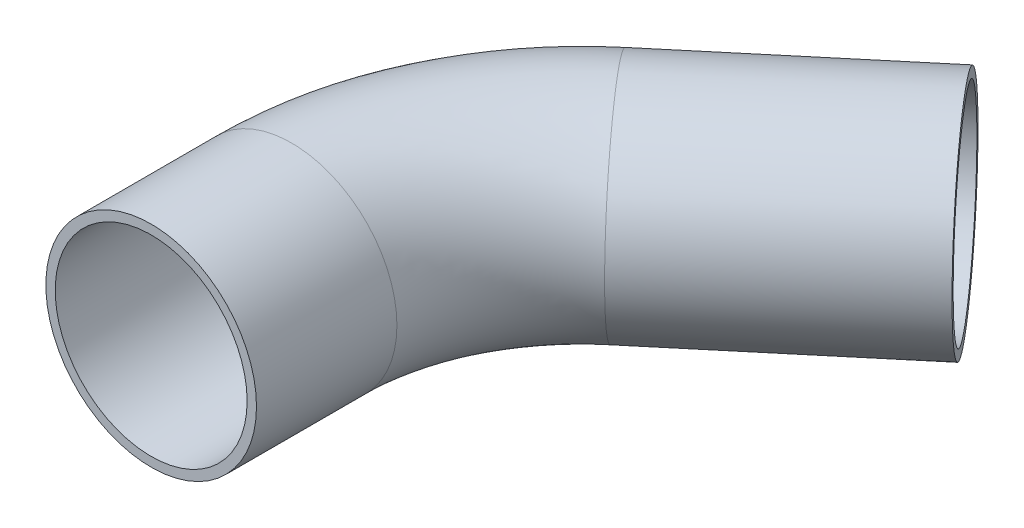
SolidWorks part; units mm, degrees
ref_plane "Front Plane" through (0, 0, 0) normal (0, 0, 1) x (1, 0, 0)
ref_plane "Top Plane" through (0, 0, 0) normal (0, 1, 0) x (1, 0, 0)
ref_plane "Right Plane" through (0, 0, 0) normal (1, 0, 0) x (0, 0, -1)
sketch "Sketch1" plane through (0, 0, 0) normal (0, 0, 1) x (1, 0, 0)
  circle A0 centre (0, 0) radius 22.5
sketch "Sketch2" plane through (0, 0, 0) normal (0, 1, 0) x (1, 0, 0)
  line L0 (0, 0) -> (0, 29.9989)
  line L3 (22.1472, 77.4937) -> (62.502, 111.3554)
  arc A0 (0, 29.9989) -> (22.1472, 77.4937) centre (62, 29.9989) cw
  dimension "D2" = 62
  dimension "D1" = 130
sweep "Sweep1" add profiles "Sketch1" path "Sketch2"
shell "Shell1" thickness 2
